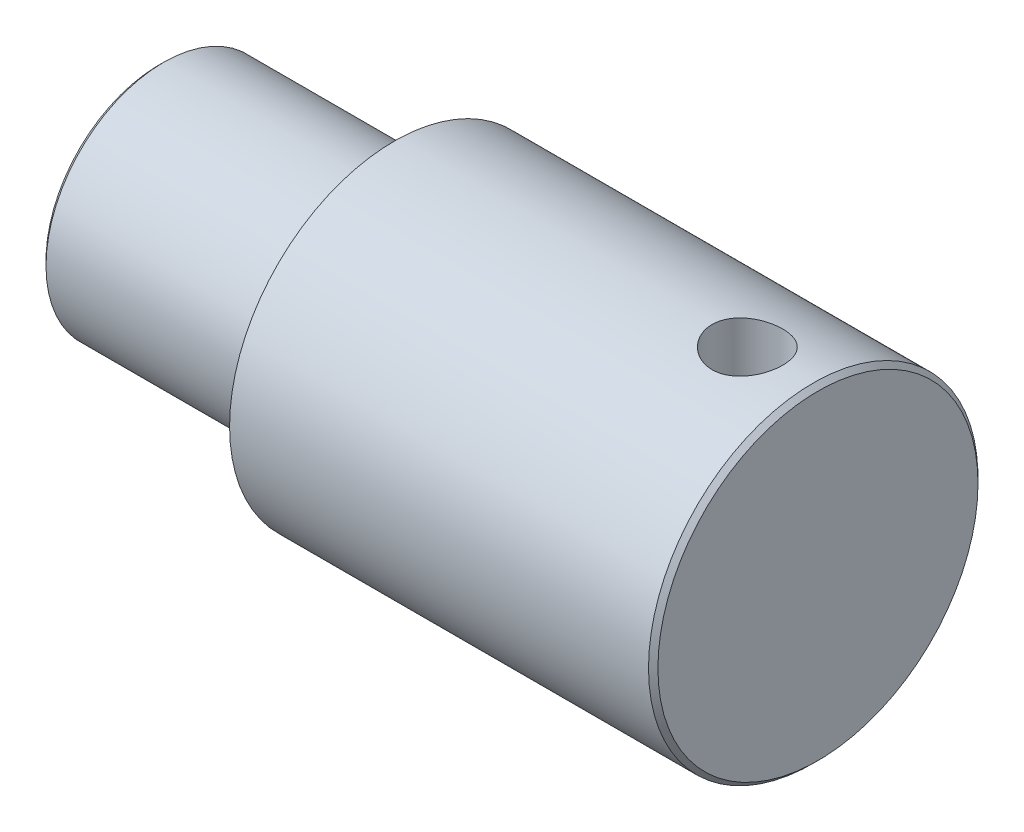
SolidWorks part; units mm, degrees
ref_plane "Front Plane" through (0, 0, 0) normal (0, 0, 1) x (1, 0, 0)
ref_plane "Top Plane" through (0, 0, 0) normal (0, 1, 0) x (1, 0, 0)
ref_plane "Right Plane" through (0, 0, 0) normal (1, 0, 0) x (0, 0, -1)
sketch "Sketch1" plane through (0, 0, 0) normal (0, 0, 1) x (1, 0, 0)
  line L0 (0, 0) -> (40.5225, 0) construction
  line L1 (0, 0) -> (0, 5)
  line L2 (0, 5) -> (10, 5)
  line L3 (10, 5) -> (10, 7)
  line L4 (10, 7) -> (28, 7)
  line L5 (28, 7) -> (28, 0)
  line L6 (28, 0) -> (0, 0)
  dimension "D1" = 10
  dimension "D2" = 14
  dimension "D3" = 18
  dimension "D4" = 10
revolve "Revolve1" add sketch "Sketch1" angle 360 about L0
chamfer "Chamfer1" distance 0.2 angle 45 1 edges at (0, 0, 5)
sketch "Sketch2" plane through (10, 0, 0) normal (-1, 0, 0) x (0, 0, 1)
  circle A0 centre (0, 0) radius 5 construction
  circle A1 centre (0, 0) radius 7
  circle A2 centre (0, 0) radius 7
  circle A3 centre (0, 0) radius 5
  dimension "D1" = 0
extrude "Cut-Extrude1" [suppressed] cut sketch "Sketch2" against normal blind 13
sketch "Sketch3" plane through (0, 0, 0) normal (0, 1, 0) x (1, 0, 0)
  line L0 (0, 0) -> (25, 0) construction
  line L1 (28, -7) -> (28, 7) construction
  circle A0 centre (25, 0) radius 1.5
  dimension "D1" = 3
  dimension "D2" = 3
extrude "Cut-Extrude2" cut sketch "Sketch3" against normal through all both and the other way through all
chamfer "Chamfer2" distance 0.2 angle 45 1 edges at (28, 0, 7)
